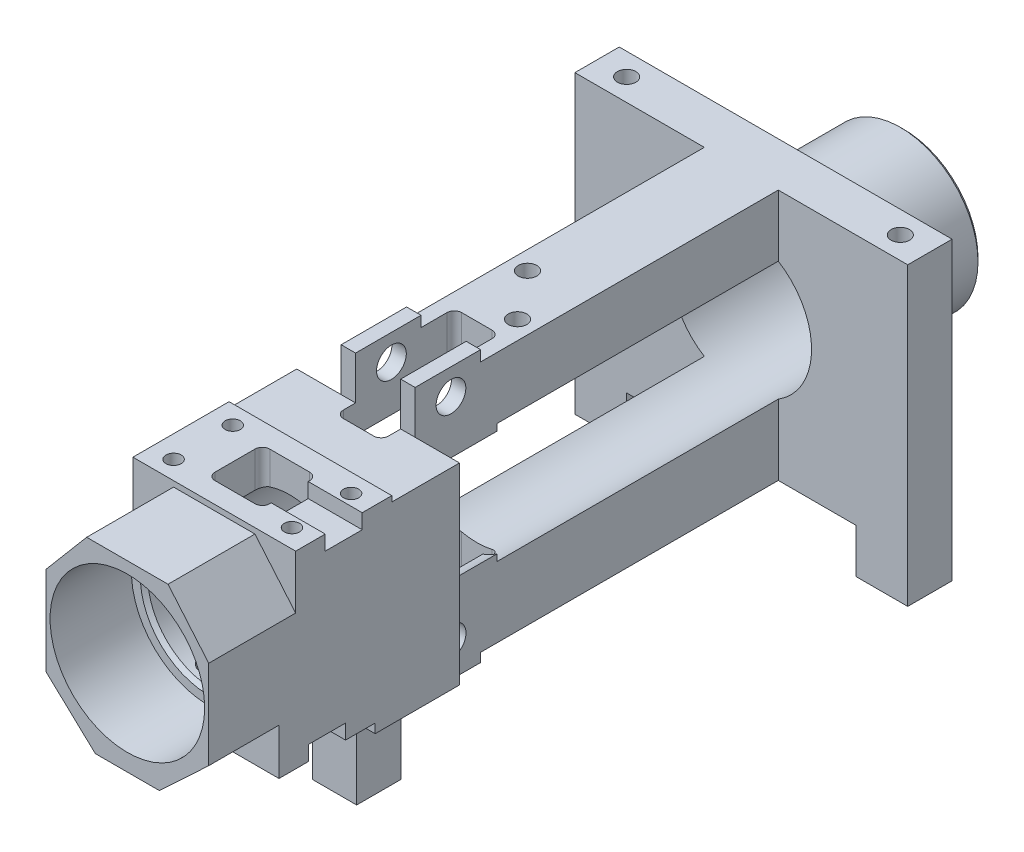
SolidWorks part; units mm, degrees
material "1060 合金"
ref_plane "前视基准面" through (0, 0, 0) normal (0, 0, 1) x (1, 0, 0)
ref_plane "上视基准面" through (0, 0, 0) normal (0, 1, 0) x (1, 0, 0)
ref_plane "右视基准面" through (0, 0, 0) normal (1, 0, 0) x (0, 0, -1)
other "质心 (COM)"
other "Configuration Table"
sketch "草图1" plane through (0, 0, 0) normal (0, 0, 1) x (1, 0, 0)
  circle A0 centre (0, 0) radius 10.5
  dimension "D1" = 21
extrude "凸台-拉伸1" add sketch "草图1" along normal blind 16
sketch "草图2" plane through (0, 0, 16) normal (0, 0, 1) x (1, 0, 0)
  line L0 (-18.5, 34.8342) -> (-18.5, -37.949) construction
  line L1 (-22.5, 16.4) -> (22.5, 16.4)
  line L2 (-22.5, 16.4) -> (-22.5, -23.6)
  line L3 (-22.5, -23.6) -> (22.5, -23.6)
  line L4 (22.5, 16.4) -> (22.5, -23.6)
  line L5 (18.5, 34.0036) -> (18.5, -37.949) construction
  dimension "D1" = 37
  dimension "D2" = 18.5
  dimension "D3" = 4
  dimension "D4" = 4
  dimension "D5" = 40
  dimension "D6" = 23.6
extrude "凸台-拉伸2" add sketch "草图2" along normal blind 6
sketch "草图3" plane through (0, 0, 22) normal (0, 0, 1) x (1, 0, 0)
  line L0 (22.5, 16.4) -> (-22.5, 16.4) construction
  line L1 (-5, 16.4) -> (5, 16.4)
  line L2 (-5, 16.4) -> (-5, -23.6)
  line L3 (-5, -23.6) -> (5, -23.6)
  line L4 (5, 16.4) -> (5, -23.6)
  line L5 (-22.5, -23.6) -> (22.5, -23.6) construction
  dimension "D1" = 10
  dimension "D2" = 5
extrude "凸台-拉伸3" add sketch "草图3" along normal blind 59
sketch "草图4" plane through (0, -23.6, 0) normal (0, -1, 0) x (1, 0, 0)
  line L0 (0, 0) -> (0, 81) construction
  line L1 (-5, 81) -> (5, 81) construction
  line L2 (-22.5, 16) -> (22.5, 16) construction
  line L5 (-18.5, 19) -> (18.5, 19) construction
  line L6 (-36.625, 52.1) -> (36.625, 52.1) construction
  line L8 (-11, 81) -> (11, 81)
  line L9 (-11, 81) -> (-11, 71.1)
  line L10 (-11, 71.1) -> (11, 71.1)
  line L11 (11, 81) -> (11, 71.1)
  circle A0 centre (-18.5, 19) radius 1.5 construction
  circle A1 centre (18.5, 19) radius 1.5 construction
  circle A2 centre (-36.625, 52.1) radius 30 construction
  circle A3 centre (36.625, 52.1) radius 30 construction
  circle A4 centre (0, 63.9684) radius 8.5 construction
  dimension "D1" = 3
  dimension "D2" = 3
  dimension "D3" = 18.5
  dimension "D7" = 60
  dimension "D10" = 17
  dimension "D4" = 11
  dimension "D5" = 36.625
  dimension "D6" = 33.1
  dimension "D8" = 11
  dimension "D9" = 19
extrude "凸台-拉伸4" add sketch "草图4" against normal up to surface (40 mm away) up to face at (0, 16.4, 35.25)
sketch "草图5" plane through (5, 0, 0) normal (1, 0, 0) x (0, 0, -1)
  line L0 (-52.1, 16.4) -> (-52.1, -23.6) construction
  line L1 (-82.1, -23.6) -> (-22.1, -23.6) construction
  line L2 (-71.1, -23.6) -> (-22, -23.6) construction
  line L3 (-71.1, 16.4) -> (-22, 16.4) construction
  line L4 (0, 0) -> (-52.1, 0) construction
  line L5 (-52.1, 0) -> (-81, 0) construction
  line L6 (-81, 16.4) -> (-81, -23.6) construction
  line L7 (-71.1, 16.4) -> (-71.1, -23.6) construction
  line L8 (-71.1, 17.84) -> (-62.25, 17.84)
  line L9 (-71.1, 17.84) -> (-71.1, 16.4)
  line L10 (-71.1, 16.4) -> (-62.25, 16.4)
  line L11 (-62.25, 17.84) -> (-62.25, 16.4)
  circle A0 centre (-66.25, 14.34) radius 2.015 construction
  circle A1 centre (-66.25, -14.34) radius 2.015 construction
  circle A2 centre (-66.25, 14.34) radius 6.5 construction
  point P4 (-52.1, -23.6)
  dimension "D1" = 14.15
  dimension "D2" = 28.68
  dimension "D3" = 4.03
  dimension "D5" = 13
  dimension "D4" = 3.5
  dimension "D6" = 4
extrude "凸台-拉伸5" add sketch "草图5" against normal up to surface (10 mm away) up to face at (-5, -3.6, 46.55)
sketch "草图6" plane through (0, 0, 81) normal (0, 0, 1) x (1, 0, 0)
  line L0 (0, 0) -> (0, -23.6) construction
  line L1 (-11, -23.6) -> (11, -23.6) construction
  circle A0 centre (0, 0) radius 8.75
  dimension "D1" = 17.5
extrude "切除-拉伸1" cut sketch "草图6" against normal through all
sketch "草图7" plane through (0, 0, 81) normal (0, 0, 1) x (1, 0, 0)
  line L0 (11, 16.4) -> (11, -23.6) construction
  line L1 (-11, 16.4) -> (11, 16.4)
  line L2 (-11, 16.4) -> (-11, 12)
  line L3 (-11, 12) -> (11, 12)
  line L4 (11, 16.4) -> (11, 12)
  line L5 (-11, 16.4) -> (-11, -23.6) construction
  line L6 (-11, -14) -> (11, -14)
  line L7 (-11, -14) -> (-11, -23.6)
  line L8 (-11, -23.6) -> (11, -23.6)
  line L9 (11, -14) -> (11, -23.6)
  dimension "D1" = 12
  dimension "D2" = 14
extrude "切除-拉伸2" cut sketch "草图7" against normal up to surface (9.9 mm away) up to face at (7.625, -2.4, 71.1)
sketch "草图8" plane through (0, 17.84, 0) normal (0, 1, 0) x (1, 0, 0)
  line L0 (0, 0) -> (0, -81) construction
  line L1 (-11, -81) -> (11, -81) construction
  line L2 (5, -52.1) -> (0, -52.1) construction
  line L3 (-5, -65.75) -> (5, -65.75) construction
  line L4 (-5, -71.1) -> (-5, -62.25) construction
  line L5 (5, -68.265) -> (5, -64.235) construction
  line L7 (-3.05, -57.75) -> (3.05, -57.75)
  line L8 (-3.05, -57.75) -> (-3.05, -73.75)
  line L9 (-3.05, -73.75) -> (3.05, -73.75)
  line L10 (3.05, -57.75) -> (3.05, -73.75)
  dimension "D1" = 13.65
  dimension "D2" = 8
  dimension "D3" = 8
  dimension "D4" = 3.05
  dimension "D5" = 3.05
extrude "切除-拉伸3" cut sketch "草图8" against normal through all
sketch "草图9" plane through (0, 0, 71.1) normal (0, 0, 1) x (1, 0, 0)
  line L0 (5, 16.4) -> (5, -23.6) construction
  line L1 (-5, -23.6) -> (5, -23.6)
  line L2 (-5, -23.6) -> (-5, -18.8)
  line L3 (-5, -18.8) -> (5, -18.8)
  line L4 (5, -23.6) -> (5, -18.8)
  dimension "D1" = 4.8
extrude "切除-拉伸4" cut sketch "草图9" against normal up to surface (13.35 mm away) up to face at (0, -16.0378, 57.75)
sketch "草图10" plane through (0, 0, 16) normal (0, 0, -1) x (-1, 0, 0)
  line L0 (22.5, -23.6) -> (-22.5, -23.6) construction
  line L1 (-15.5, -23.6) -> (15.5, -23.6)
  line L2 (-15.5, -23.6) -> (-15.5, -17.6)
  line L3 (-15.5, -17.6) -> (15.5, -17.6)
  line L4 (15.5, -23.6) -> (15.5, -17.6)
  line L5 (-22.5, -23.6) -> (-22.5, 16.4) construction
  line L6 (22.5, 16.4) -> (22.5, -23.6) construction
  dimension "D1" = 6
  dimension "D2" = 7
  dimension "D3" = 7
extrude "切除-拉伸5" cut sketch "草图10" against normal blind 29.4
sketch "草图11" plane through (0, -23.6, 0) normal (0, -1, 0) x (1, 0, 0)
  line L0 (5, 57.75) -> (-5, 57.75) construction
  line L1 (5, 45.4) -> (-5, 45.4) construction
  line L2 (-5, 57.75) -> (-5, 45.4) construction
  line L3 (5, 0) -> (5, 52.1) construction
  line L4 (-22.5, 22) -> (-22.5, 16) construction
  line L5 (-22.5, 16) -> (-15.5, 16) construction
  circle A0 centre (-2.5, 54.75) radius 1.25 construction
  circle A1 centre (2.5, 48.4) radius 1.25 construction
  circle A2 centre (-18.5, 19) radius 1.25 construction
  circle A3 centre (18.5, 19) radius 1.25 construction
  dimension "D1" = 3
  dimension "D2" = 3
  dimension "D3" = 2.5
  dimension "D4" = 2.5
  dimension "D5" = 2.5
  dimension "D6" = 2.5
  dimension "D7" = 2.5
  dimension "D8" = 2.5
  dimension "D9" = 37
  dimension "D10" = 4
  dimension "D11" = 3
hole_wizard "M3 螺纹孔1" positions "草图12" profile "草图13" tap size "M3" standard "GB"
sketch "草图12" plane through (0, -23.6, 0) normal (0, -1, 0) x (-1, 0, 0)
  point P0 (-18.5, -19)
  point P3 (18.5, -19)
  point P6 (-2.5, -48.4)
  point P9 (2.5, -54.75)
sketch "草图13" plane through (18.5, -23.6, 19) normal (1, 0, 0) x (0, 0, -1)
  line L0 (0, 0) -> (0, 5.7511)
  line L1 (0, 5.7511) -> (1.25, 5)
  line L2 (1.25, 5) -> (1.25, 0)
  line L5 (1.25, 0) -> (0, 0)
  line L10 (0, 5.7511) -> (-1.25, 5) construction
  line L11 (0, -6.35) -> (0, 107.95) construction
  dimension "螺纹孔钻头直径" = 2.5
  dimension "螺纹孔钻头深度" = 5
  dimension "导头角度" = 118
cosmetic thread "孔螺蚊线1" parameters "D1"=6, "D2"=3
cosmetic thread "孔螺蚊线2" parameters "D1"=6, "D2"=3
cosmetic thread "孔螺蚊线3" parameters "D1"=6, "D2"=3
cosmetic thread "孔螺蚊线4" parameters "D1"=6, "D2"=3
sketch "草图14" plane through (5, 0, 0) normal (1, 0, 0) x (0, 0, -1)
  circle A0 centre (-66.25, 14.34) radius 2.01
  circle A1 centre (-66.25, -14.34) radius 2.03
  dimension "D1" = 4.02
  dimension "D2" = 4.06
extrude "切除-拉伸6" cut sketch "草图14" against normal up to surface (10 mm away) up to face at (-5, 13.5488, 54.5429)
sketch "草图15" plane through (0, 16.4, 0) normal (0, 1, 0) x (1, 0, 0)
  circle A0 centre (-18.5, -19) radius 1.25 construction
  circle A1 centre (18.5, -19) radius 1.25 construction
  circle A2 centre (-2.5, -48.4) radius 1.25 construction
  circle A3 centre (2.5, -54.75) radius 1.25 construction
  dimension "D1" = 2.5
  dimension "D2" = 2.5
  dimension "D3" = 2.5
  dimension "D4" = 2.5
hole_wizard "M3 螺纹孔2" positions "草图16" profile "草图17" tap size "M3" standard "GB"
sketch "草图16" plane through (0, 16.4, 0) normal (0, 1, 0) x (1, 0, 0)
  point P0 (-18.5, -19)
  point P3 (18.5, -19)
  point P6 (-2.5, -48.4)
  point P9 (2.5, -54.75)
sketch "草图17" plane through (-18.5, 16.4, 19) normal (1, 0, 0) x (0, 0, 1)
  line L0 (0, 0) -> (0, 5.7511)
  line L1 (0, 5.7511) -> (1.25, 5)
  line L2 (1.25, 5) -> (1.25, 0)
  line L5 (1.25, 0) -> (0, 0)
  line L10 (0, 5.7511) -> (-1.25, 5) construction
  line L11 (0, -6.35) -> (0, 107.95) construction
  dimension "螺纹孔钻头直径" = 2.5
  dimension "螺纹孔钻头深度" = 5
  dimension "导头角度" = 118
cosmetic thread "孔螺蚊线5" parameters "D1"=6, "D2"=3
cosmetic thread "孔螺蚊线6" parameters "D1"=6, "D2"=3
cosmetic thread "孔螺蚊线7" parameters "D1"=6, "D2"=3
cosmetic thread "孔螺蚊线8" parameters "D1"=6, "D2"=3
sketch "草图18" plane through (0, 0, 0) normal (0, 0, -1) x (-1, 0, 0)
  circle A0 centre (0, 0) radius 9.5
  dimension "D1" = 19
extrude "切除-拉伸7" cut sketch "草图18" against normal blind 60
chamfer "倒角1" distance 0.5 angle 45 1 edges at (10.5, 0, 0)
fillet "圆角1" radius 1 1 edges at (10.5, 0, 16)
fillet "圆角2" radius 1 8 edges at (3.05, -11.1006, 73.75) (-3.05, -11.1006, 73.75) (3.05, -13.8985, 57.75) (-3.05, -13.8985, 57.75) (3.05, 12.6985, 57.75) (-3.05, 12.6985, 57.75) (3.05, 10.1006, 73.75) (-3.05, 10.1006, 73.75)
sketch "草图19" plane through (5, 0, 0) normal (1, 0, 0) x (0, 0, -1)
  circle A0 centre (-66.25, 14.34) radius 4.25 construction
  circle A1 centre (-66.25, -14.34) radius 4.25 construction
  dimension "D1" = 8.5
  dimension "D2" = 8.5
chamfer "倒角2" [suppressed] distance 2.5 distance2 10
chamfer "倒角6" [suppressed] distance 10 distance2 2.5
sketch "草图20" [suppressed] plane through (0, 0, 81) normal (0, 0, 1) x (1, 0, 0)
  line L4 (11, 12) -> (-11, 12)
  line L5 (-11, 12) -> (-11, -14)
  line L6 (-11, -14) -> (11, -14)
  line L7 (11, -14) -> (11, 12)
  line L8 (11, 12) -> (-11, 12)
  line L9 (-11, 12) -> (-11, -14)
  line L10 (-11, -14) -> (11, -14)
  line L11 (11, -14) -> (11, 12)
  circle A0 centre (0, 0) radius 8.75 construction
  circle A1 centre (0, 0) radius 8.75
  dimension "D1" = 0
extrude "凸台-拉伸6" [suppressed] add sketch "草图20" along normal blind 17
sketch "草图22" [suppressed] plane through (0, 0, 98) normal (0, 0, 1) x (1, 0, 0)
  circle A0 centre (0, 0) radius 9.75
  circle A1 centre (0, 0) radius 8.75 construction
  circle A2 centre (0, 0) radius 8.75
  dimension "D1" = 19.5
extrude "凸台-拉伸7" [suppressed] add sketch "草图22" along normal blind 8.5
chamfer "倒角4" [suppressed] distance 0.25 angle 45
sketch "草图23" [suppressed] plane through (11, 0, 0) normal (1, 0, 0) x (0, 0, -1)
  line L0 (0, 0) -> (-120.3408, 0) construction
sketch "草图24" plane through (0, -23.6, 0) normal (0, -1, 0) x (-1, 0, 0)
  line L0 (-5, -62.25) -> (5, -62.25)
  line L3 (5, -45.4) -> (-5, -45.4)
  line L4 (-5, -62.25) -> (-5, -45.4)
  line L5 (5, -57.75) -> (5, -71.1) construction
  line L6 (5, -62.25) -> (5, -45.4)
  line L7 (5, -62.25) -> (3.05, -62.25) construction
extrude "切除-拉伸8" cut sketch "草图24" against normal up to surface (6 mm away) up to face at (0, -17.6, 26.35)
sketch "草图25" plane through (0, 0, 81) normal (0, 0, 1) x (1, 0, 0)
  line L8 (-11, -14) -> (11, -14)
  line L10 (11, -14) -> (11, 12)
  line L12 (11, 12) -> (-11, 12)
  line L14 (-11, 12) -> (-11, -14)
  line L16 (-11, -14) -> (11, -14)
  line L18 (11, -14) -> (11, 12)
  line L20 (11, 12) -> (-11, 12)
  line L22 (-11, 12) -> (-11, -14)
  circle A0 centre (0, 0) radius 8.75
  dimension "D1" = 17.5
  dimension "D3" = 0
extrude "凸台-拉伸8" add sketch "草图25" along normal blind 24
sketch "草图26" plane through (0, 0, 105) normal (0, 0, 1) x (1, 0, 0)
  circle A0 centre (0, 0) radius 10.45
  dimension "D1" = 20.9
extrude "切除-拉伸9" cut sketch "草图26" against normal blind 11
chamfer "倒角5" distance 0.5 angle 45 1 edges at (8.75, 0, 94)
sketch "草图27" plane through (0, -14, 0) normal (0, -1, 0) x (-1, 0, 0)
  line L0 (0, 0) -> (0, -128.5449) construction
  line L1 (8.5, -76.5) -> (8.5, -82.5)
  line L3 (8.5, -82.5) -> (2.5, -82.5)
  line L4 (8.5, -76.5) -> (2.5, -76.5)
  line L7 (2.5, -82.5) -> (2.5, -76.5)
  line L11 (-8.5, -76.5) -> (-2.5, -76.5)
  line L12 (-2.5, -82.5) -> (-2.5, -76.5)
  line L13 (-8.5, -82.5) -> (-2.5, -82.5)
  line L14 (-8.5, -76.5) -> (-8.5, -82.5)
  circle A0 centre (5.5, -79.5) radius 1.2
  circle A1 centre (18.5, -19) radius 1.25 construction
  circle A2 centre (18.5, -19) radius 1.25 construction
  circle A3 centre (-5.5, -79.5) radius 1.2
  circle A4 centre (5.5, -79.5) radius 3 construction
  dimension "D1" = 60.5
  dimension "D2" = 13
  dimension "D3" = 2.4
  dimension "D4" = 6
extrude "凸台-拉伸9" add sketch "草图27" along normal up to surface (9.6 mm away) up to face at (-18.5, -23.6, 17.75)
hole_wizard "M3 螺纹孔5" positions "草图40" profile "草图39" tap size "M3" standard "GB"
sketch "草图40" plane through (0, -23.6, 0) normal (0, -1, 0) x (-1, 0, 0)
  point P0 (-5.5, -79.5)
  point P3 (5.5, -79.5)
sketch "草图39" plane through (5.5, -23.6, 79.5) normal (1, 0, 0) x (0, 0, -1)
  line L0 (0, 0) -> (0, 10.3511)
  line L1 (0, 10.3511) -> (1.25, 9.6)
  line L2 (1.25, 9.6) -> (1.25, 0)
  line L5 (1.25, 0) -> (0, 0)
  line L10 (0, 10.3511) -> (-1.25, 9.6) construction
  line L11 (0, -6.35) -> (0, 107.95) construction
  dimension "螺纹孔钻头直径" = 2.5
  dimension "螺纹孔钻头深度" = 9.6
  dimension "导头角度" = 118
cosmetic thread "孔螺纹线5" parameters "D1"=4.5, "D2"=3
cosmetic thread "孔螺纹线6" parameters "D1"=4.5, "D2"=3
sketch "草图41" plane through (0, 12, 0) normal (0, 1, 0) x (1, 0, 0)
  line L0 (0, -86.009) -> (0, 49913.991) construction
  line L1 (-11, -80.25) -> (11, -80.25)
  line L2 (-11, -80.25) -> (-11, -93.25)
  line L3 (-11, -93.25) -> (11, -93.25)
  line L4 (11, -80.25) -> (11, -93.25)
  line L5 (-11, -80.25) -> (11, -93.25) construction
  line L6 (-11, -93.25) -> (11, -80.25) construction
  line L7 (0, -86.75) -> (50000, -86.75) construction
  line L9 (5, -71.1) -> (11, -71.1) construction
  line L10 (11, -71.1) -> (11, -105) construction
  line L11 (-2.7, -90.45) -> (2.7, -90.45)
  line L12 (-3.7, -89.45) -> (-3.7, -84.05)
  line L13 (-2.7, -83.05) -> (2.7, -83.05)
  line L14 (3.7, -89.45) -> (3.7, -84.05)
  line L15 (-3.7, -90.45) -> (3.7, -83.05) construction
  line L16 (-3.7, -83.05) -> (3.7, -90.45) construction
  circle A0 centre (-8, -82.75) radius 1
  circle A1 centre (8, -82.75) radius 1
  circle A2 centre (-8, -90.75) radius 1
  circle A3 centre (8, -90.75) radius 1
  arc A8 (2.7, -90.45) -> (3.7, -89.45) centre (2.7, -89.45) ccw
  arc A9 (-2.7, -90.45) -> (-3.7, -89.45) centre (-2.7, -89.45) cw
  arc A10 (-3.7, -84.05) -> (-2.7, -83.05) centre (-2.7, -84.05) cw
  arc A11 (2.7, -83.05) -> (3.7, -84.05) centre (2.7, -84.05) cw
  point P0 (0, -86.75)
  point P32 (0, -86.75)
  dimension "D3" = 8
  dimension "D4" = 16
  dimension "D5" = 2
  dimension "D9" = 1
  dimension "D1" = 13
  dimension "D6" = 15.65
  dimension "D8" = 7.4
extrude "顶部灯板定位" add sketch "草图41" along normal offset from surface (0.75 mm away) 0.75 up to face at (0, 12, 77.5012) offset beyond the face yes
sketch "草图44" plane through (0, 12, 0) normal (0, 1, 0) x (1, 0, 0)
  line L4 (-2.7, -90.45) -> (2.7, -90.45)
  line L5 (3.7, -89.45) -> (3.7, -84.05)
  line L6 (2.7, -83.05) -> (-2.7, -83.05)
  line L7 (-3.7, -84.05) -> (-3.7, -89.45)
  line L8 (-2.7, -90.45) -> (2.7, -90.45)
  line L9 (3.7, -89.45) -> (3.7, -84.05)
  line L10 (2.7, -83.05) -> (-2.7, -83.05)
  line L11 (-3.7, -84.05) -> (-3.7, -89.45)
  arc A4 (2.7, -90.45) -> (3.7, -89.45) centre (2.7, -89.45) ccw
  arc A5 (3.7, -84.05) -> (2.7, -83.05) centre (2.7, -84.05) ccw
  arc A6 (-2.7, -83.05) -> (-3.7, -84.05) centre (-2.7, -84.05) ccw
  arc A7 (-3.7, -89.45) -> (-2.7, -90.45) centre (-2.7, -89.45) ccw
  arc A8 (2.7, -90.45) -> (3.7, -89.45) centre (2.7, -89.45) ccw
  arc A9 (3.7, -84.05) -> (2.7, -83.05) centre (2.7, -84.05) ccw
  arc A10 (-2.7, -83.05) -> (-3.7, -84.05) centre (-2.7, -84.05) ccw
  arc A11 (-3.7, -89.45) -> (-2.7, -90.45) centre (-2.7, -89.45) ccw
  dimension "D1" = 0
extrude "顶部灯珠留空" cut sketch "草图44" against normal up to vertex (12 mm away) up to point (0, 0, 0)
hole_wizard "顶部灯板固定孔" positions "草图45" profile "草图46" tap size "M2.5" standard "GB"
sketch "草图45" plane through (0, 12.75, 0) normal (0, 1, 0) x (1, 0, 0)
  point P0 (-8, -82.75)
  point P3 (8, -82.75)
  point P6 (8, -90.75)
  point P9 (-8, -90.75)
sketch "草图46" plane through (-8, 12.75, 82.75) normal (1, 0, 0) x (0, 0, 1)
  line L0 (0, 0) -> (0, 6.8159)
  line L1 (0, 6.8159) -> (1.025, 6.2)
  line L2 (1.025, 6.2) -> (1.025, 0)
  line L5 (1.025, 0) -> (0, 0)
  line L10 (0, 6.8159) -> (-1.025, 6.2) construction
  line L11 (0, -6.35) -> (0, 107.95) construction
  dimension "螺纹孔钻头直径" = 2.05
  dimension "螺纹孔钻头深度" = 6.2
  dimension "导头角度" = 118
cosmetic thread "孔螺纹线7" parameters "D1"=5, "D2"=2.5
cosmetic thread "孔螺纹线8" parameters "D1"=5, "D2"=2.5
cosmetic thread "孔螺纹线9" parameters "D1"=5, "D2"=2.5
cosmetic thread "孔螺纹线10" parameters "D1"=5, "D2"=2.5
sketch "草图51" plane through (0, 12.75, 0) normal (0, 1, 0) x (1, 0, 0)
  line L0 (6.8006, -86.75) -> (50006.8006, -86.75) construction
  line L1 (3.7, -89.25) -> (11, -89.25)
  line L2 (3.7, -89.25) -> (3.7, -84.25)
  line L3 (3.7, -84.25) -> (11, -84.25)
  line L4 (11, -89.25) -> (11, -84.25)
  line L5 (3.7, -89.25) -> (11, -84.25) construction
  line L6 (3.7, -84.25) -> (11, -89.25) construction
  line L7 (3.7, -84.05) -> (3.7, -89.45) construction
  line L8 (-11, -80.25) -> (11, -80.25) construction
  line L9 (-11, -93.25) -> (11, -93.25) construction
  line L10 (11, -71.1) -> (11, -80.25) construction
  point P0 (7.35, -86.75)
  dimension "D1" = 5
extrude "顶部焊点留空" cut sketch "草图51" against normal blind 2
sketch "草图47" plane through (0, -14, 0) normal (0, -1, 0) x (-1, 0, 0)
  line L0 (0, -88.259) -> (0, 49911.741) construction
  line L1 (-11.5, -82.5) -> (11.5, -82.5)
  line L2 (-12.5, -83.5) -> (-12.5, -94.5)
  line L3 (-11.5, -95.5) -> (11.5, -95.5)
  line L4 (12.5, -83.5) -> (12.5, -94.5)
  line L5 (-12.5, -82.5) -> (12.5, -95.5) construction
  line L6 (-12.5, -95.5) -> (12.5, -82.5) construction
  line L7 (0, -89) -> (50000, -89) construction
  line L10 (8.5, -82.5) -> (2.5, -82.5) construction
  line L11 (-2.7, -92.7) -> (2.7, -92.7)
  line L12 (-3.7, -91.7) -> (-3.7, -86.3)
  line L13 (-2.7, -85.3) -> (2.7, -85.3)
  line L14 (3.7, -91.7) -> (3.7, -86.3)
  line L15 (-3.7, -92.7) -> (3.7, -85.3) construction
  line L16 (-3.7, -85.3) -> (3.7, -92.7) construction
  circle A0 centre (-8, -85) radius 1
  circle A1 centre (8, -85) radius 1
  circle A2 centre (-8, -93) radius 1
  circle A3 centre (8, -93) radius 1
  arc A4 (-12.5, -94.5) -> (-11.5, -95.5) centre (-11.5, -94.5) ccw
  arc A5 (11.5, -95.5) -> (12.5, -94.5) centre (11.5, -94.5) ccw
  arc A6 (11.5, -82.5) -> (12.5, -83.5) centre (11.5, -83.5) cw
  arc A7 (-11.5, -82.5) -> (-12.5, -83.5) centre (-11.5, -83.5) ccw
  arc A8 (2.7, -92.7) -> (3.7, -91.7) centre (2.7, -91.7) ccw
  arc A9 (-2.7, -92.7) -> (-3.7, -91.7) centre (-2.7, -91.7) cw
  arc A10 (-3.7, -86.3) -> (-2.7, -85.3) centre (-2.7, -86.3) cw
  arc A11 (2.7, -85.3) -> (3.7, -86.3) centre (2.7, -86.3) cw
  point P0 (0, -89)
  point P32 (0, -89)
  dimension "D3" = 8
  dimension "D4" = 16
  dimension "D5" = 2
  dimension "D7" = 1
  dimension "D9" = 1
  dimension "D1" = 13
  dimension "D2" = 25
  dimension "D8" = 7.4
extrude "底部灯板定位" cut sketch "草图47" against normal offset from surface (1.25 mm away) 1.25 up to face at (5.5, -14, 79.5)
sketch "草图50" plane through (0, -14, 0) normal (0, -1, 0) x (1, 0, 0)
  line L4 (-3.7, 91.7) -> (-3.7, 86.3)
  line L5 (-2.7, 85.3) -> (2.7, 85.3)
  line L6 (3.7, 86.3) -> (3.7, 91.7)
  line L7 (2.7, 92.7) -> (-2.7, 92.7)
  line L8 (-3.7, 91.7) -> (-3.7, 86.3)
  line L9 (-2.7, 85.3) -> (2.7, 85.3)
  line L10 (3.7, 86.3) -> (3.7, 91.7)
  line L11 (2.7, 92.7) -> (-2.7, 92.7)
  arc A4 (-2.7, 92.7) -> (-3.7, 91.7) centre (-2.7, 91.7) ccw
  arc A5 (-3.7, 86.3) -> (-2.7, 85.3) centre (-2.7, 86.3) ccw
  arc A6 (2.7, 85.3) -> (3.7, 86.3) centre (2.7, 86.3) ccw
  arc A7 (3.7, 91.7) -> (2.7, 92.7) centre (2.7, 91.7) ccw
  arc A8 (-2.7, 92.7) -> (-3.7, 91.7) centre (-2.7, 91.7) ccw
  arc A9 (-3.7, 86.3) -> (-2.7, 85.3) centre (-2.7, 86.3) ccw
  arc A10 (2.7, 85.3) -> (3.7, 86.3) centre (2.7, 86.3) ccw
  arc A11 (3.7, 91.7) -> (2.7, 92.7) centre (2.7, 91.7) ccw
  dimension "D1" = 0
extrude "底部灯珠留空" cut sketch "草图50" against normal up to vertex up to point (0, 0, 0)
hole_wizard "底部灯板固定孔" positions "草图48" profile "草图49" tap size "M2.5" standard "GB"
sketch "草图48" plane through (0, -14, 0) normal (0, -1, 0) x (-1, 0, 0)
  point P0 (-8, -85)
  point P3 (8, -85)
  point P5 (8, -93)
  point P8 (-8, -93)
sketch "草图49" plane through (8, -14, 85) normal (1, 0, 0) x (0, 0, -1)
  line L0 (0, 0) -> (0, 6.9659)
  line L1 (0, 6.9659) -> (1.025, 6.35)
  line L2 (1.025, 6.35) -> (1.025, 0)
  line L5 (1.025, 0) -> (0, 0)
  line L10 (0, 6.9659) -> (-1.025, 6.35) construction
  line L11 (0, -6.35) -> (0, 107.95) construction
  dimension "螺纹孔钻头直径" = 2.05
  dimension "螺纹孔钻头深度" = 6.35
  dimension "导头角度" = 118
cosmetic thread "孔螺纹线11" parameters "D1"=5, "D2"=2.5
cosmetic thread "孔螺纹线12" parameters "D1"=5, "D2"=2.5
cosmetic thread "孔螺纹线13" parameters "D1"=5, "D2"=2.5
cosmetic thread "孔螺纹线14" parameters "D1"=5, "D2"=2.5
sketch "草图52" plane through (0, -12.75, 0) normal (0, -1, 0) x (1, 0, 0)
  line L0 (3.7, 86.3) -> (3.7, 91.7) construction
  line L1 (11, 86.5) -> (3.7, 86.5)
  line L2 (11, 86.5) -> (11, 91.5)
  line L3 (11, 91.5) -> (3.7, 91.5)
  line L4 (3.7, 86.5) -> (3.7, 91.5)
  line L5 (11, 86.5) -> (3.7, 91.5) construction
  line L6 (11, 91.5) -> (3.7, 86.5) construction
  line L7 (11, 71.1) -> (11, 82.5) construction
  line L8 (7.35, 89) -> (50007.35, 89) construction
  line L9 (-11, 82.5) -> (11, 82.5) construction
  line L10 (11, 95.5) -> (-11, 95.5) construction
  point P0 (7.35, 89)
  dimension "D1" = 5
extrude "底部焊点留空" cut sketch "草图52" against normal blind 2 and the other way through all
sketch "草图53" plane through (0, 0, 105) normal (0, 0, 1) x (1, 0, 0)
  line L0 (-5.5, 12) -> (-11, 5.5)
  line L1 (-11, 12) -> (-5.5, 12)
  line L2 (-11, 12) -> (-11, 5.5)
  line L3 (-11, -14) -> (-3, -14)
  line L5 (-11, -6.5) -> (-3, -14)
  line L9 (-11, -6.5) -> (-11, -14)
  line L12 (0, 0) -> (0, -50000) construction
  line L13 (-11, -14) -> (11, -14) construction
  line L14 (11, -6.5) -> (11, -14)
  line L15 (11, -6.5) -> (3, -14)
  line L16 (11, -14) -> (3, -14)
  line L17 (11, 12) -> (11, 5.5)
  line L18 (5.5, 12) -> (11, 5.5)
  line L19 (11, 12) -> (5.5, 12)
  line L20 (-4.3333, -12.75) -> (4.3333, -12.75)
  line L21 (-3, -14) -> (3, -14)
  line L24 (6.975, -12.75) -> (9.025, -12.75) construction
  line M15 (11, -14) -> (11, 12)
  line M16 (11, 12) -> (-11, 12)
  line M17 (-11, 12) -> (-11, -14)
  line M18 (-11, -14) -> (11, -14)
  dimension "D1" = 5.5
  dimension "D2" = 6.5
  dimension "D3" = 8
  dimension "D4" = 7.5
extrude "减重镂空1" cut sketch "草图53" against normal up to surface (9.5 mm away) contours L20 L12 L21 L15 | L12 L20 L5 M18 | L15 M15 M18 | L5 M17 M18 | L18 M16 M15 | L0 M16 M17 up to face at (0, -13.375, 95.5)
sketch "草图54" plane through (0, 0, 95.5) normal (0, 0, 1) x (1, 0, 0)
  line L0 (11, 12) -> (5.5, 12) construction
  line L1 (5.5, 12) -> (11, 5.5) construction
  line L2 (11, 5.5) -> (11, 12) construction
  line L3 (-11, 12) -> (-11, 5.5) construction
  line L4 (-11, 5.5) -> (-5.5, 12) construction
  line L5 (-5.5, 12) -> (-11, 12) construction
  line L6 (11, 12) -> (5.5, 12)
  line L7 (5.5, 12) -> (11, 5.5)
  line L8 (11, 5.5) -> (11, 12)
  line L9 (-11, 12) -> (-11, 5.5)
  line L10 (-11, 5.5) -> (-5.5, 12)
  line L11 (-5.5, 12) -> (-11, 12)
extrude "减重镂空2" cut sketch "草图54" against normal up to surface (2.25 mm away) up to face at (0, 12.375, 93.25)
